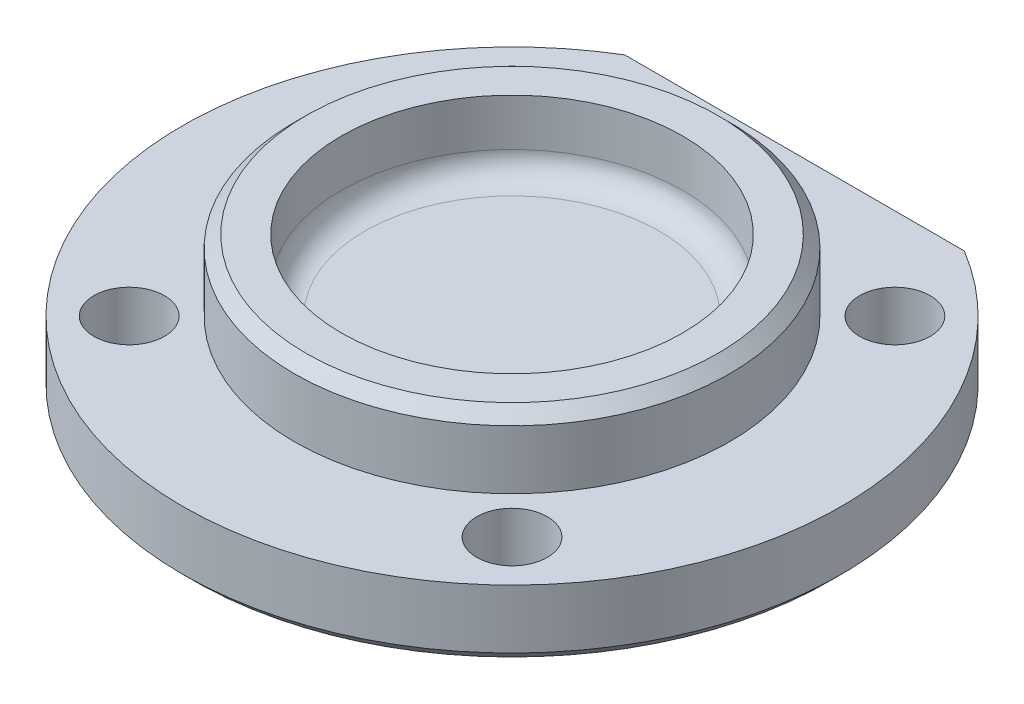
SolidWorks part; units mm, degrees
ref_plane "Front Plane" through (0, 0, 0) normal (0, 0, 1) x (1, 0, 0)
ref_plane "Top Plane" through (0, 0, 0) normal (0, 1, 0) x (1, 0, 0)
ref_plane "Right Plane" through (0, 0, 0) normal (1, 0, 0) x (0, 0, -1)
other "Configuration Table"
sketch "Sketch1" plane through (0, 0, 0) normal (0, 1, 0) x (1, 0, 0)
  circle A0 centre (0, 0) radius 28
  dimension "D1" = 56
extrude "Boss-Extrude1" add sketch "Sketch1" along normal blind 6
sketch "Sketch2" plane through (0, 6, 0) normal (0, 1, 0) x (1, 0, 0)
  circle A0 centre (0, 0) radius 18.5
  dimension "D1" = 37
extrude "Boss-Extrude2" add sketch "Sketch2" along normal blind 6
sketch "Sketch3" plane through (0, 12, 0) normal (0, 1, 0) x (1, 0, 0)
  circle A0 centre (0, 0) radius 14.5
  dimension "D1" = 29
extrude "Cut-Extrude1" cut sketch "Sketch3" against normal blind 6
fillet "Fillet2" radius 2 1 edges at (0, 6, 14.5)
chamfer "Chamfer1" distance 1 angle 45 2 edges at (0, 0, 28) (0, 12, 18.5)
sketch "Sketch4" plane through (0, 6, 0) normal (0, 1, 0) x (1, 0, 0)
  line L0 (0, 35.2194) -> (0, 0) construction
  line L1 (0, 0) -> (-16.2635, 16.2635) construction
  circle A0 centre (0, 0) radius 23 construction
  circle A1 centre (-16.2635, 16.2635) radius 3
  circle A5 centre (16.2635, 16.2635) radius 3
  circle A6 centre (16.2635, -16.2635) radius 3
  circle A7 centre (-16.2635, -16.2635) radius 3
  point P14 (-0.111, -1.8971)
  point P15 (0, 0)
  dimension "D1" = 46
  dimension "D2" = 6
  dimension "D4" = 45
  dimension "D3" = 4
extrude "Cut-Extrude2" cut sketch "Sketch4" against normal blind 6
sketch "Sketch5" plane through (0, 6, 0) normal (0, 1, 0) x (1, 0, 0)
  line L1 (-21.2121, 31.7069) -> (26.9339, 31.7069)
  line L2 (-21.2121, 31.7069) -> (-21.2121, 24)
  line L3 (-21.2121, 24) -> (26.9339, 24)
  line L4 (26.9339, 31.7069) -> (26.9339, 24)
  line L5 (-21.2121, 31.7069) -> (26.9339, 24) construction
  line L6 (-21.2121, 24) -> (26.9339, 31.7069) construction
  circle A0 centre (0, 0) radius 28 construction
  point P0 (2.8609, 27.8535)
  dimension "D1" = 24
extrude "Cut-Extrude3" cut sketch "Sketch5" against normal blind 6
